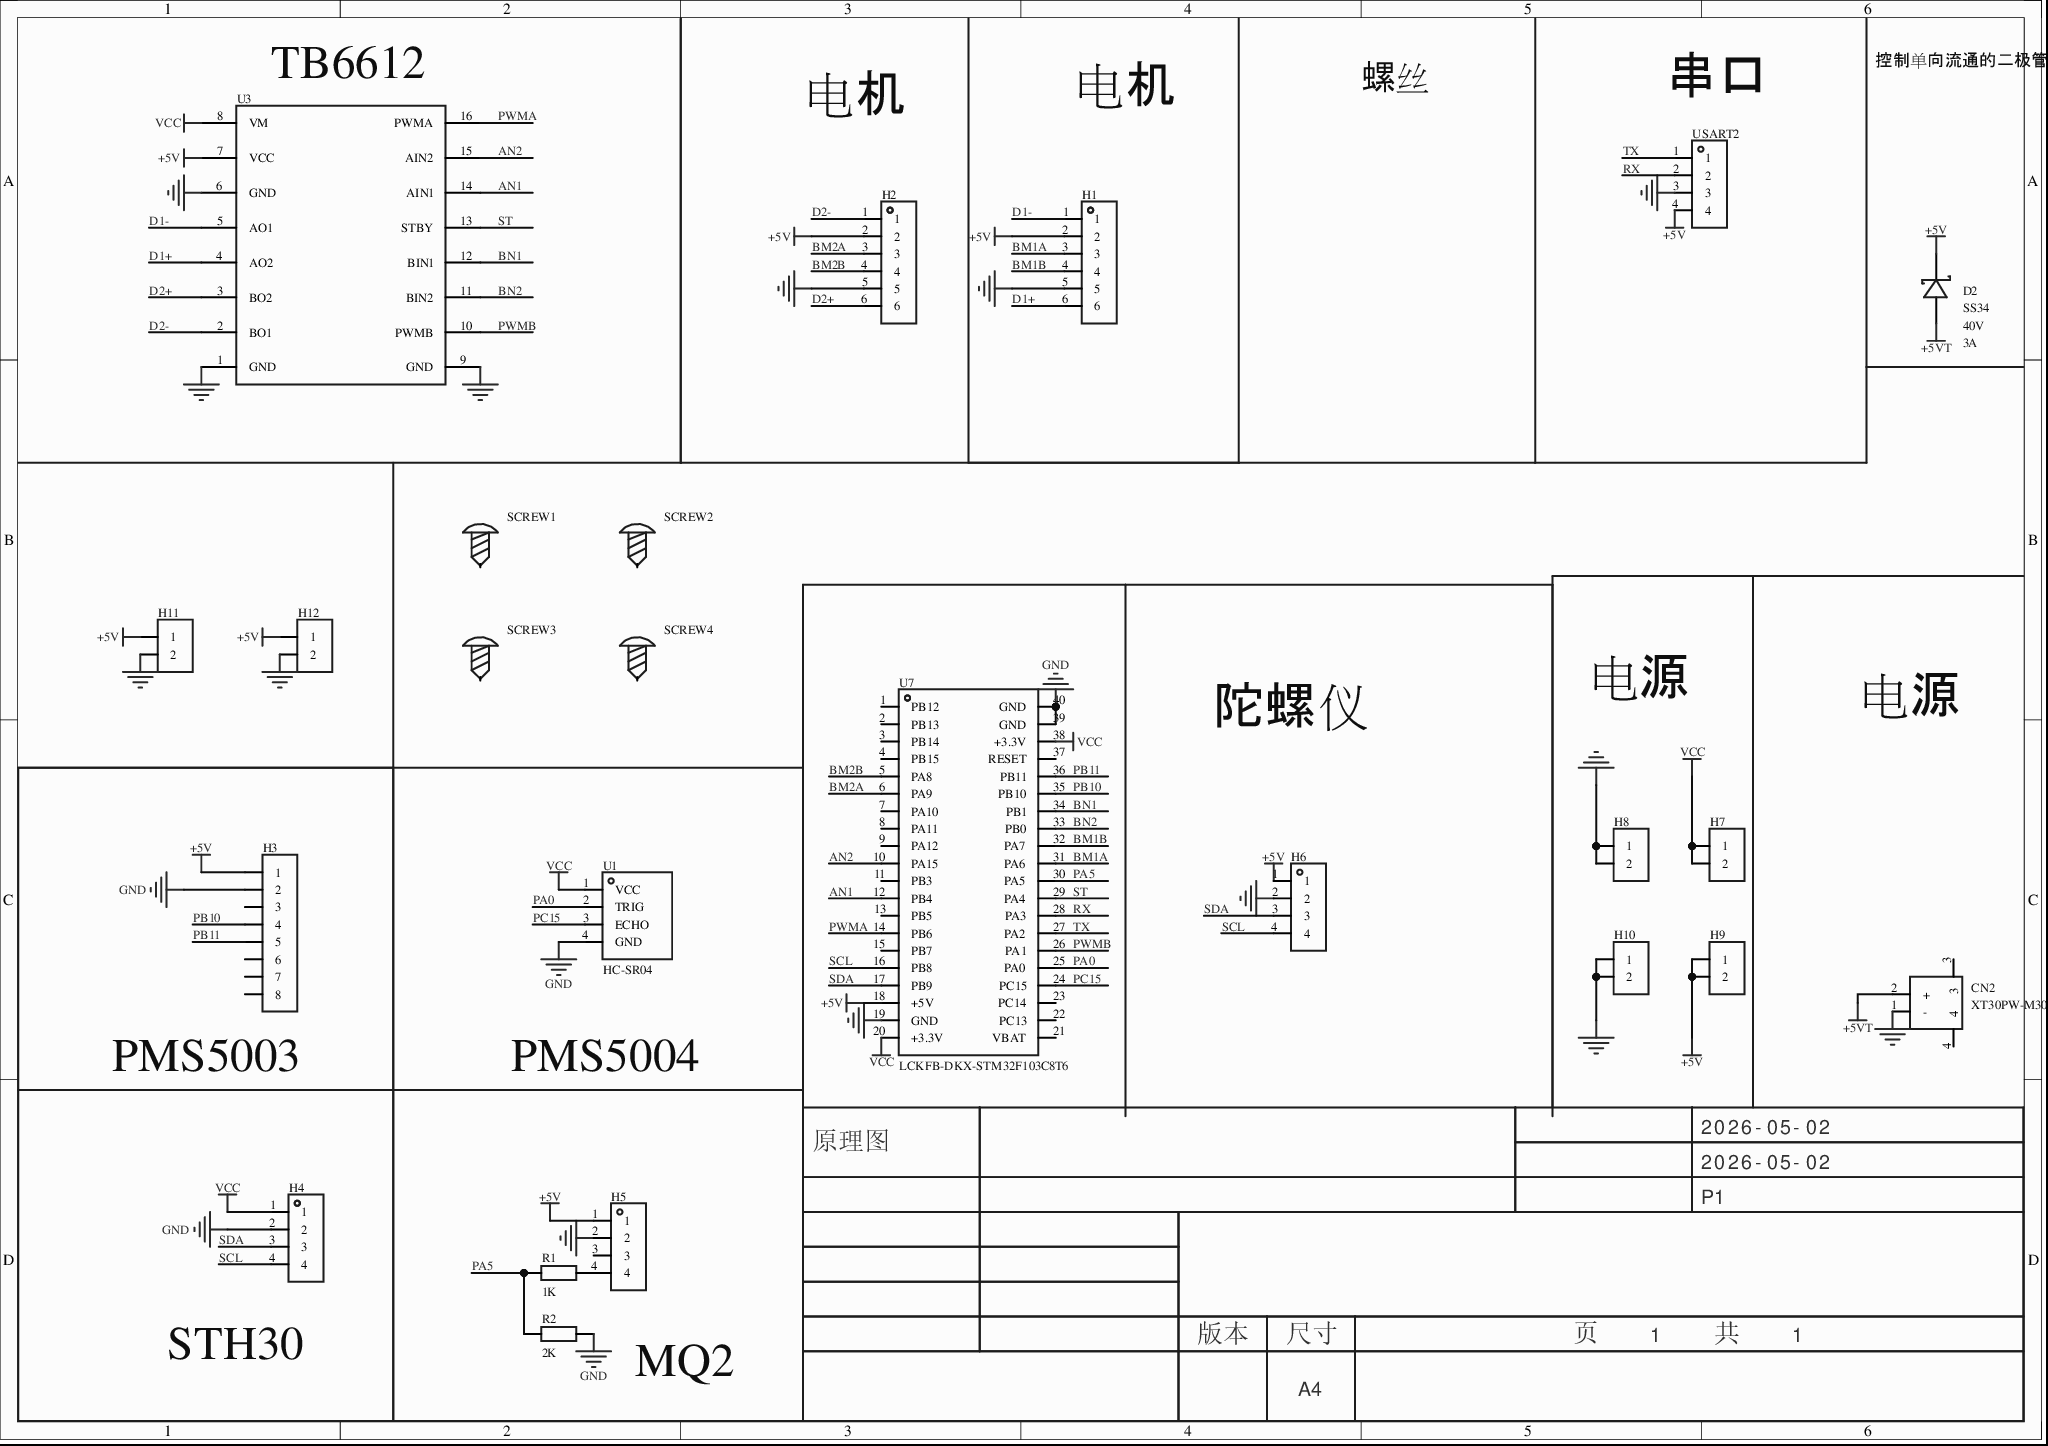
[diagram p0: MISC52026-3.schdoc]
# Altium project MISC52026-2.PrjPcb
1 sheet, 24 parts. Net scope: global (net labels, ports and power ports of the same name join across sheets).
Board file: MISC52026.pcbdoc

## Sheet MISC52026-3.schdoc
size 297 x 209 mm; Version: V1.0; @Project Name: MISC52026; @Page Count: 1; @Update Date: 2026-05-02; @Create Date: 2026-05-02; @Schematic Name: MISC52026; @Page No: 1; @Create Time: 07:27:29; @Update Time: 12:01:53; @Board Name: MISC52026

### Parts
CN2  XT30PW-M30.G.Y  [CONN-TH_XT30PW-M]
D2  SS34  Reverse Voltage (Vr): 40V  Rectified Current: 3A  [SMC_L6.9-W5.9-LS7.9-RD]
H1  (no value)  [HDR-TH_6P-P2.54-V-F]
H2  (no value)  [HDR-TH_6P-P2.54-V-F]
H3  (no value)  [HDR-TH_8P-P2.54-V-F-1]
H4  (no value)  [HDR-TH_4P-P2.54-V-F]
H5  (no value)  [HDR-TH_4P-P2.54-V-M]
H6  (no value)  [HDR-TH_4P-P2.54-V-M]
H7  (no value)  [HDR-TH_2P-P2.54-V-F]
H8  (no value)  [HDR-TH_2P-P2.54-V-F]
H9  (no value)  [HDR-TH_2P-P2.54-V-F]
H10  (no value)  [HDR-TH_2P-P2.54-V-F]
H11  (no value)  [HDR-TH_2P-P2.54-V-F]
H12  (no value)  [HDR-TH_2P-P2.54-V-F]
R1  1K  [R0603]
R2  2K  [R0603]
SCREW1  (no value)  [M2螺丝]
SCREW2  (no value)  [M2螺丝]
SCREW3  (no value)  [M2螺丝]
SCREW4  (no value)  [M2螺丝]
U1  HC-SR04  [TH_HC-SR04V]
U3  (no value)  [TB6612]
U7  LCKFB-DKX-STM32F103C8T6  [CONN-TH_L53.3-W22.9_STM32F103C8T6-CARD]
USART2  (no value)  [HDR-TH_4P-P2.54-V-M]

### Blocks framed on the sheet
PMS5003: H3
PMS5004: U1
STH30: H4
MQ2: H5 R1 R2

### Nets
+5V: D2.1(C) H1.2 H2.2 H3.1 H5.1 H6.1 H9.1 H9.2 H11.1 H12.1 U3.7(VCC) U7.18(+5V) USART2.4
+5VT: CN2.2(+) D2.2(A)
GND: CN2.1(-) H1.5 H2.5 H3.2 H4.2 H5.2 H6.2 H8.1 H8.2 H10.1 H10.2 H11.2 H12.2 R2.2 U1.4(GND) U3.1(GND) U3.6(GND) U3.9(GND) U7.19(GND) U7.39(GND) U7.40(GND) USART2.3
VCC: H4.1 H7.1 H7.2 U1.1(VCC) U3.8(VM) U7.20(+3.3V) U7.38(+3.3V)
AN1: U3.14(AIN1) U7.12(PB4)
AN2: U3.15(AIN2) U7.10(PA15)
BM1A: H1.3 U7.31(PA6)
BM1B: H1.4 U7.32(PA7)
BM2A: H2.3 U7.6(PA9)
BM2B: H2.4 U7.5(PA8)
BN1: U3.12(BIN1) U7.34(PB1)
BN2: U3.11(BIN2) U7.33(PB0)
D1+: H1.6 U3.4(AO2)
D1-: H1.1 U3.5(AO1)
D2+: H2.6 U3.3(BO2)
D2-: H2.1 U3.2(BO1)
PA0: U1.2(TRIG) U7.25(PA0)
PA5: R1.1 R2.1 U7.30(PA5)
PB10: H3.4 U7.35(PB10)
PB11: H3.5 U7.36(PB11)
PC15: U1.3(ECHO) U7.24(PC15)
PWMA: U3.16(PWMA) U7.14(PB6)
PWMB: U3.10(PWMB) U7.26(PA1)
RX: U7.28(PA3) USART2.2
SCL: H4.4 H6.4 U7.16(PB8)
SDA: H4.3 H6.3 U7.17(PB9)
ST: U3.13(STBY) U7.29(PA4)
TX: U7.27(PA2) USART2.1
NetH5_4: H5.4 R1.2

Not connected (* = marked no-connect by the designer): CN2 3* 4*; H3 3 6 7 8; H5 3; SCREW1 1; SCREW2 1; SCREW3 1; SCREW4 1; U7 1(PB12)* 2(PB13)* 3(PB14)* 4(PB15)* 7(PA10)* 8(PA11)* 9(PA12)* 11(PB3)* 13(PB5)* 15(PB7)* 21(VBAT)* 22(PC13)* 23(PC14)* 37(RESET)*

### Notes on the sheet
- (near U3) TB6612
- 控制单向流通的二极管
- 电机
- 螺丝
- (near USART2) 串口
- 陀螺仪
- 电源
- 串口：
  PMS5003（5V供电）    ------------------  PB10， PB11   （串口3）
  ze07-co    -------------- 单独弄出来他的引脚即可 不用供电 不用连GND
  这个模块需要引出的引脚有 VCC GND TX RX
  我要用杜邦线把 VCC GND TX RX与别的主控板连接
  IIC：
  sth30（3.3V供电）    ----------- SDA->PB9    SCL->PB8
  ADC：
  mq2 （5V供电）       ----------    AO->PA6  用电阻分压：1kΩ + 2kΩ 分压（或类似比例），把最高5V降到3.3V以内接入ADC
  GPIO：
  US100（3.3V供电）    ----------   TRIG->PA0   ECHO->PA7
  把PAO PA7 VCC GND 单独引出来 需要供电 需要连GND
  只不过我要用杜邦线把PAO PA7 VCC GND与US100模块连接
- 2026-05-02
- 原理图
- P1
- 版本
- 尺寸
- A4
- 页    1    共    1

### Library data of the parts
CN2 = XT30PW-M30.G.Y: 类别:-;类型1:-;; Manufacturer: AMASS(艾迈斯); AddInBom: yes; ModelId: 722652c2597f41cd937322584dc4b29b; ModelTransform: 523.621,549.2115,0,0,0,0,-0.005,-39.568,-78.74; RatedVoltage: DC 500V; InterfaceType: 公头; RatedCurrent: 15A; RecommendedWireGauge: 16/18/20AWG; contact resistance: 1.2mΩ; specifications: 2pin; Symbol: XT30PW-M; Device: XT30PW-M30.G.Y; LCSC Part Name: AMASS(艾迈斯)航模插头 卧式弯脚 XT30PW-M公头; SupplierPart: C431092; ManufacturerPart: XT30PW-M30.G.Y; Supplier Footprint: -; JLCPCB Part Class: 扩展库; Datasheet: https://atta.szlcsc.com/upload/public/pdf/source/20220222/6A9F22F7850E25B33E1BE430ADF8560B.pdf; Supplier: LCSC; ConvertToPcb: yes; FootprintName: CONN-TH_XT30PW-M; ModelName: CONN-TH_XT30PW-M; Power: -; Output: -; Input: -; Size: -; Interface: -; Type: 航模插头; Colour: -; MaximumCurrent: -; Type1: -; NumberOfUSBHoles: -; MetalMaterial: -; InsulationMaterial: -; FlameRetardantGrade: -; Belt length: -
D2 = SS34_C154551: 正向压降(Vf):500mV@3A;直流反向耐压(Vr):40V;整流电流:3A;; Manufacturer: onsemi(安森美); AddInBom: yes; ModelId: 4f14ab132b494223bc17c7f39616ac35; ModelTransform: 314.96,236.22,0,0,0,0,0,0,0; Reverse Leakage Current (Ir): 500uA@40V; Symbol: SS34_C154551; Device: SS34_C154551; LCSC Part Name: 电压:40V 电流:3A; SupplierPart: C154551; ManufacturerPart: SS34; Supplier Footprint: SMC(DO-214AB); JLCPCB Part Class: Extended Part; Datasheet: https://atta.szlcsc.com/upload/public/pdf/source/20230523/C977B907190B075B30FD168351032A84.pdf; Supplier: LCSC; ConvertToPcb: yes; FootprintName: SMC_L6.9-W5.9-LS7.9-RD; ModelName: SMC_L6.9-W5.9-LS7.9-RD; Forward Voltage (Vf@If): 500mV@3A
H1 H2 = HDR-F_2.54_1x6P: Symbol: Header-Female-2.54_1x6; ConvertToPcb: yes; ModelId: 0f5bcf94dcda47d085f24cdca1696fe9; ModelTransform: 619.684,94.488,0,0,0,0,0,0,-125.984; Device: HDR-F_2.54_1x6P; AddInBom: yes; SupplierPart: C40877; Supplier Footprint: 插件; FootprintName: HDR-TH_6P-P2.54-V-F; ModelName: HDR-TH_6P-P2.54-V-F
H3 = HDR-F_2.54_1x8P: Symbol: Header-Female-2.54_1x8; AddInBom: yes; ModelId: 0f7e4d9227ef4fa08d5469c22cc70cdb; ModelName: HDR-F-2.54_1x8; ModelTransform: 799.99844,100,0,0,0,0,0,0,-118.11; Device: HDR-F_2.54_1x8P; ConvertToPcb: yes; FootprintName: HDR-TH_8P-P2.54-V-F-1; SupplierPart: C27438; Supplier Footprint: 插件
H4 = HDR-F_2.54_1x4P: Symbol: 2.54-1*4P母; 3D Model: d187812051054f85879fcaa51a310d8e; 3D Model Transform: 419.6842,98.464,0,0,0,0,0,0,-118.11; ConvertToPcb: yes; Device: HDR-F_2.54_1x4P; Supplier Part: C2718488; Supplier Footprint: 插件; AddInBom: yes; FootprintName: HDR-TH_4P-P2.54-V-F; ModelName: HDR-TH_4P-P2.54-V-F
H5 = HDR-M_2.54_1x4P: Symbol: PZ254V-11-04P; 3D Model: 112f4d05e8d64e99ab9a333894bea4f9; 3D Model Transform: 399.999,104.7242,0,0,0,0,0,0,-118.11; ConvertToPcb: yes; ModelName: HDR-TH_4P-P2.54-M-LI-1X4P; Device: HDR-M_2.54_1x4P; Supplier Part: C492403; Supplier Footprint: 插件; AddInBom: yes; FootprintName: HDR-TH_4P-P2.54-V-M
H6 USART2 = HDR-M_2.54_1x4P: Symbol: PZ254V-11-04P; ConvertToPcb: yes; ModelId: 112f4d05e8d64e99ab9a333894bea4f9; ModelName: HDR-TH_4P-P2.54-M-LI-1X4P; ModelTransform: 399.999,104.7242,0,0,0,0,0,0,-118.11; Device: HDR-M_2.54_1x4P; AddInBom: yes; SupplierPart: C492403; Supplier Footprint: 插件; FootprintName: HDR-TH_4P-P2.54-V-M
H7-H12 = HDR-F_2.54_1x2P: Symbol: Header-Female-2.54_1x2; ConvertToPcb: yes; ModelId: a9450ef445564560a104363b9aacde4e; ModelName: HDR-TH_2P-P2.54-F-LI-1X2P; ModelTransform: 215.7476,98.425,0,0,0,0,0,0,-129.921; Device: HDR-F_2.54_1x2P; AddInBom: yes; SupplierPart: C49661; Supplier Footprint: 插件; FootprintName: HDR-TH_2P-P2.54-V-F
R1 R2 = Res_0603: Symbol: 电阻; ConvertToPcb: yes; ModelId: fc143cca1e79419f9cd78b61e9279f080819f05c4eef4c71ace90d822a990e87; ModelTransform: 31.8897,63.7794,0,90,0,0,0,0,0; Device: Res_0603; AddInBom: yes; Supplier Footprint: 0603; FootprintName: R0603; ModelName: R0603
  R1: Value: 1K
  R2: Value: 2K
SCREW1-SCREW4 = M2螺丝: Symbol: 螺丝孔; ConvertToPcb: yes; Device: M2螺丝; AddInBom: yes; Supplier Footprint: 插件; FootprintName: M2螺丝
U1 = HC-SR04: Manufacturer: Universal Microelectronics; AddInBom: yes; Symbol: HC-SR04; Device: HC-SR04; LCSC Part Name: HC-SR04; SupplierPart: C19857336; ManufacturerPart: HC-SR04; Supplier Footprint: -; JLCPCB Part Class: Extended Part; Datasheet: https://item.szlcsc.com/datasheet/HC-SR04/21184790.html; Supplier: LCSC; ConvertToPcb: yes; FootprintName: TH_HC-SR04V
U3 = TB6612: AddInBom: yes; Device: TB6612; SymbolName: TB6612; ConvertToPcb: yes; FootprintName: TB6612
U7 = LCKFB-DKX-STM32F103C8T6: Manufacturer: 立创开发板; AddInBom: yes; ModelId: 12c257eccf3b4e5baa9346e6693d8ea4; Symbol: LCKFB-DKX-STM32F103C8T6; Device: LCKFB-DKX-STM32F103C8T6; LCSC Part Name: 立创·地阔星-STM32F103C8T6开发板; SupplierPart: C22396880; ManufacturerPart: LCKFB-DKX-STM32F103C8T6; Supplier Footprint: -; JLCPCB Part Class: Extended Part; Datasheet: https://atta.szlcsc.com/upload/public/pdf/source/20240801/7EEF69F7480DF7C6DA98696664D658D4.pdf; Supplier: LCSC; ConvertToPcb: yes; FootprintName: CONN-TH_L53.3-W22.9_STM32F103C8T6-CARD; ModelName: CONN-TH_L53.3-W22.9_STM32F103C8T6-CARD